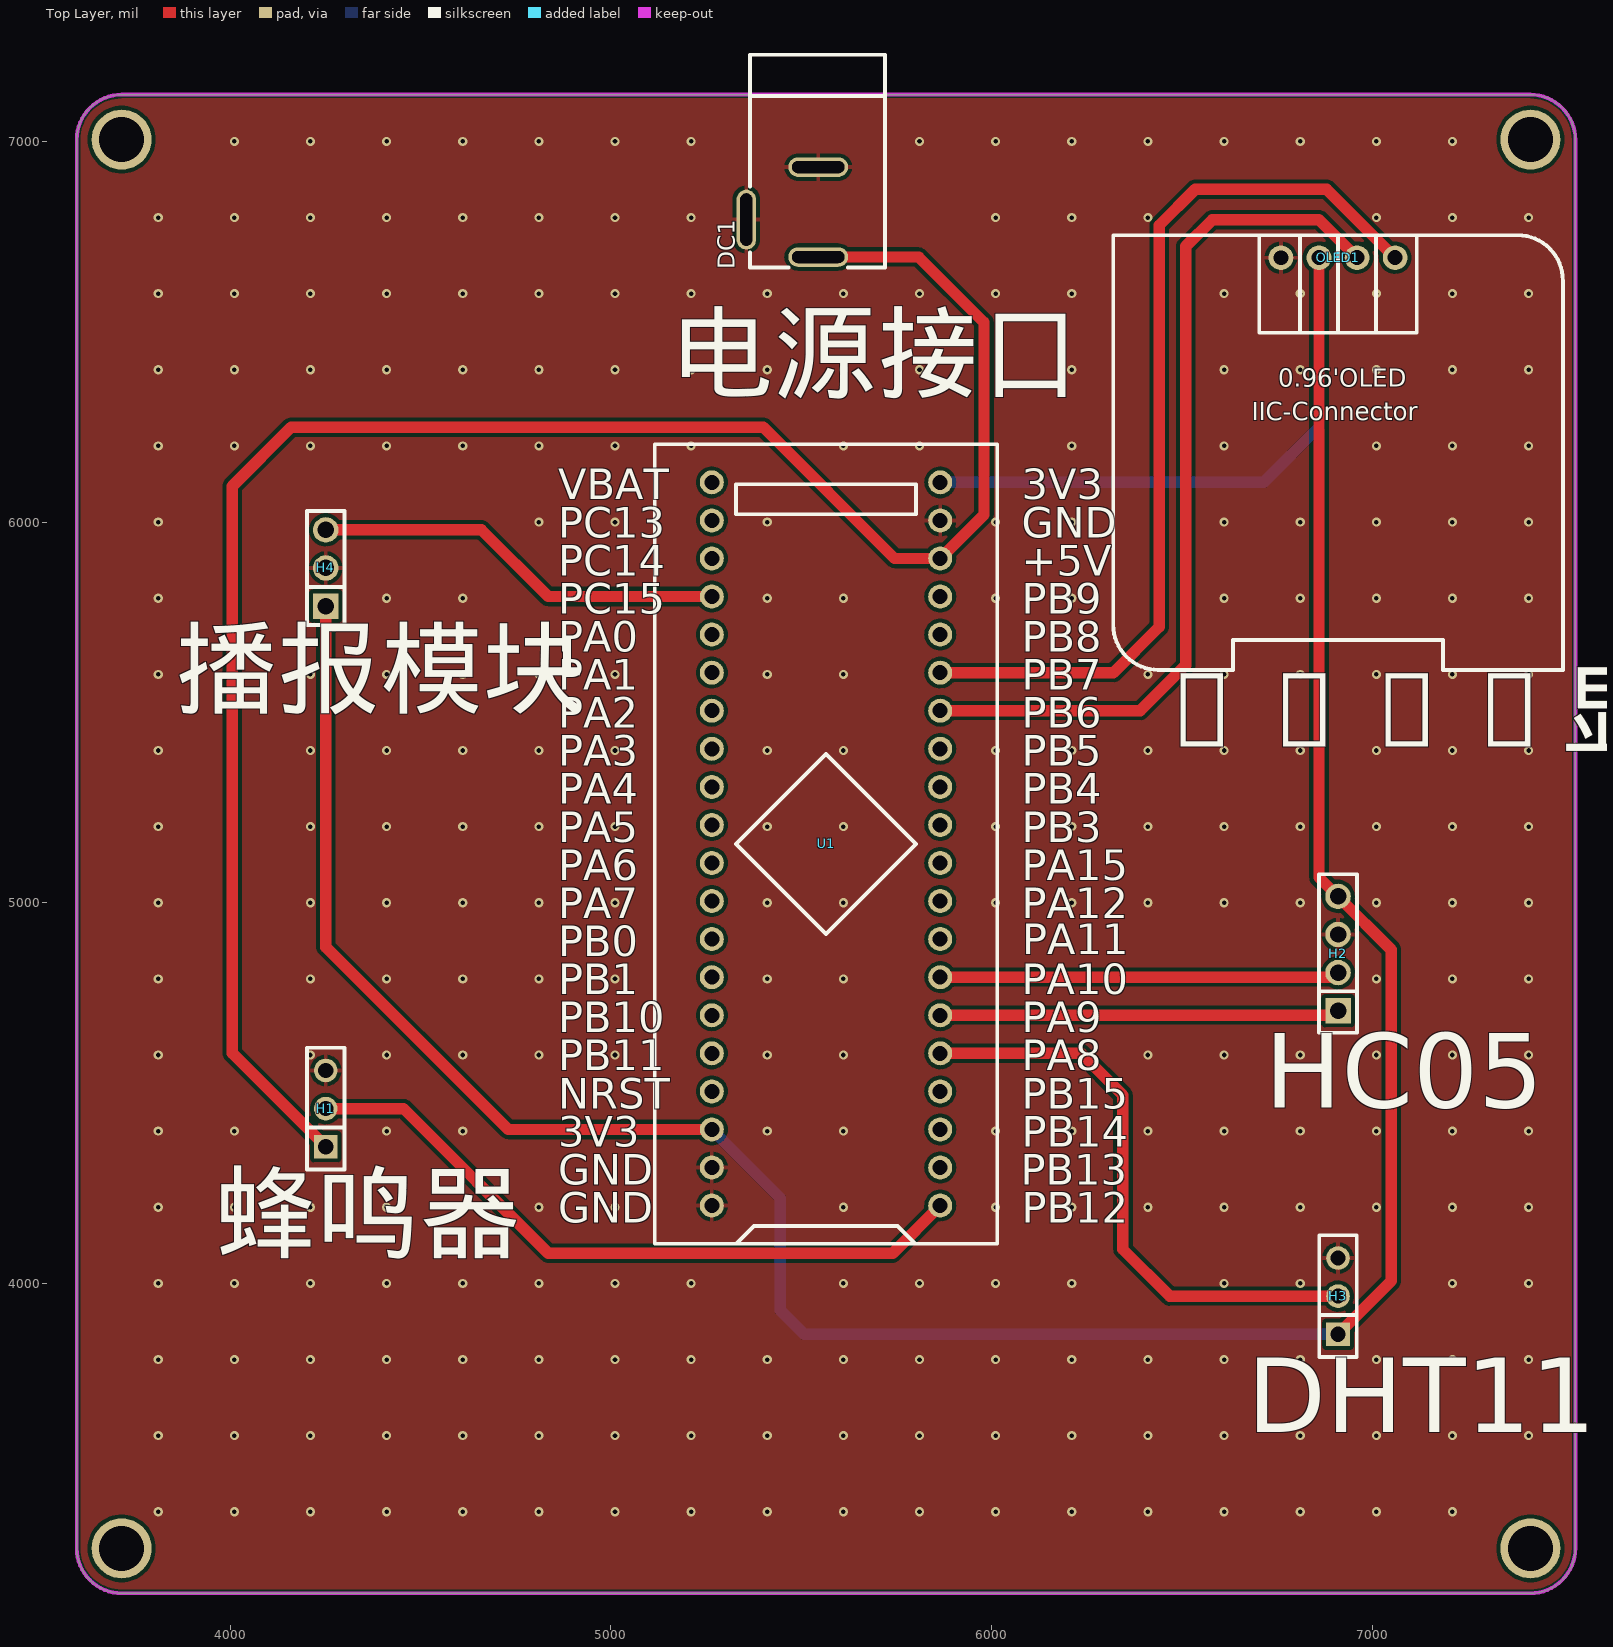
[diagram p0: Top Layer view]
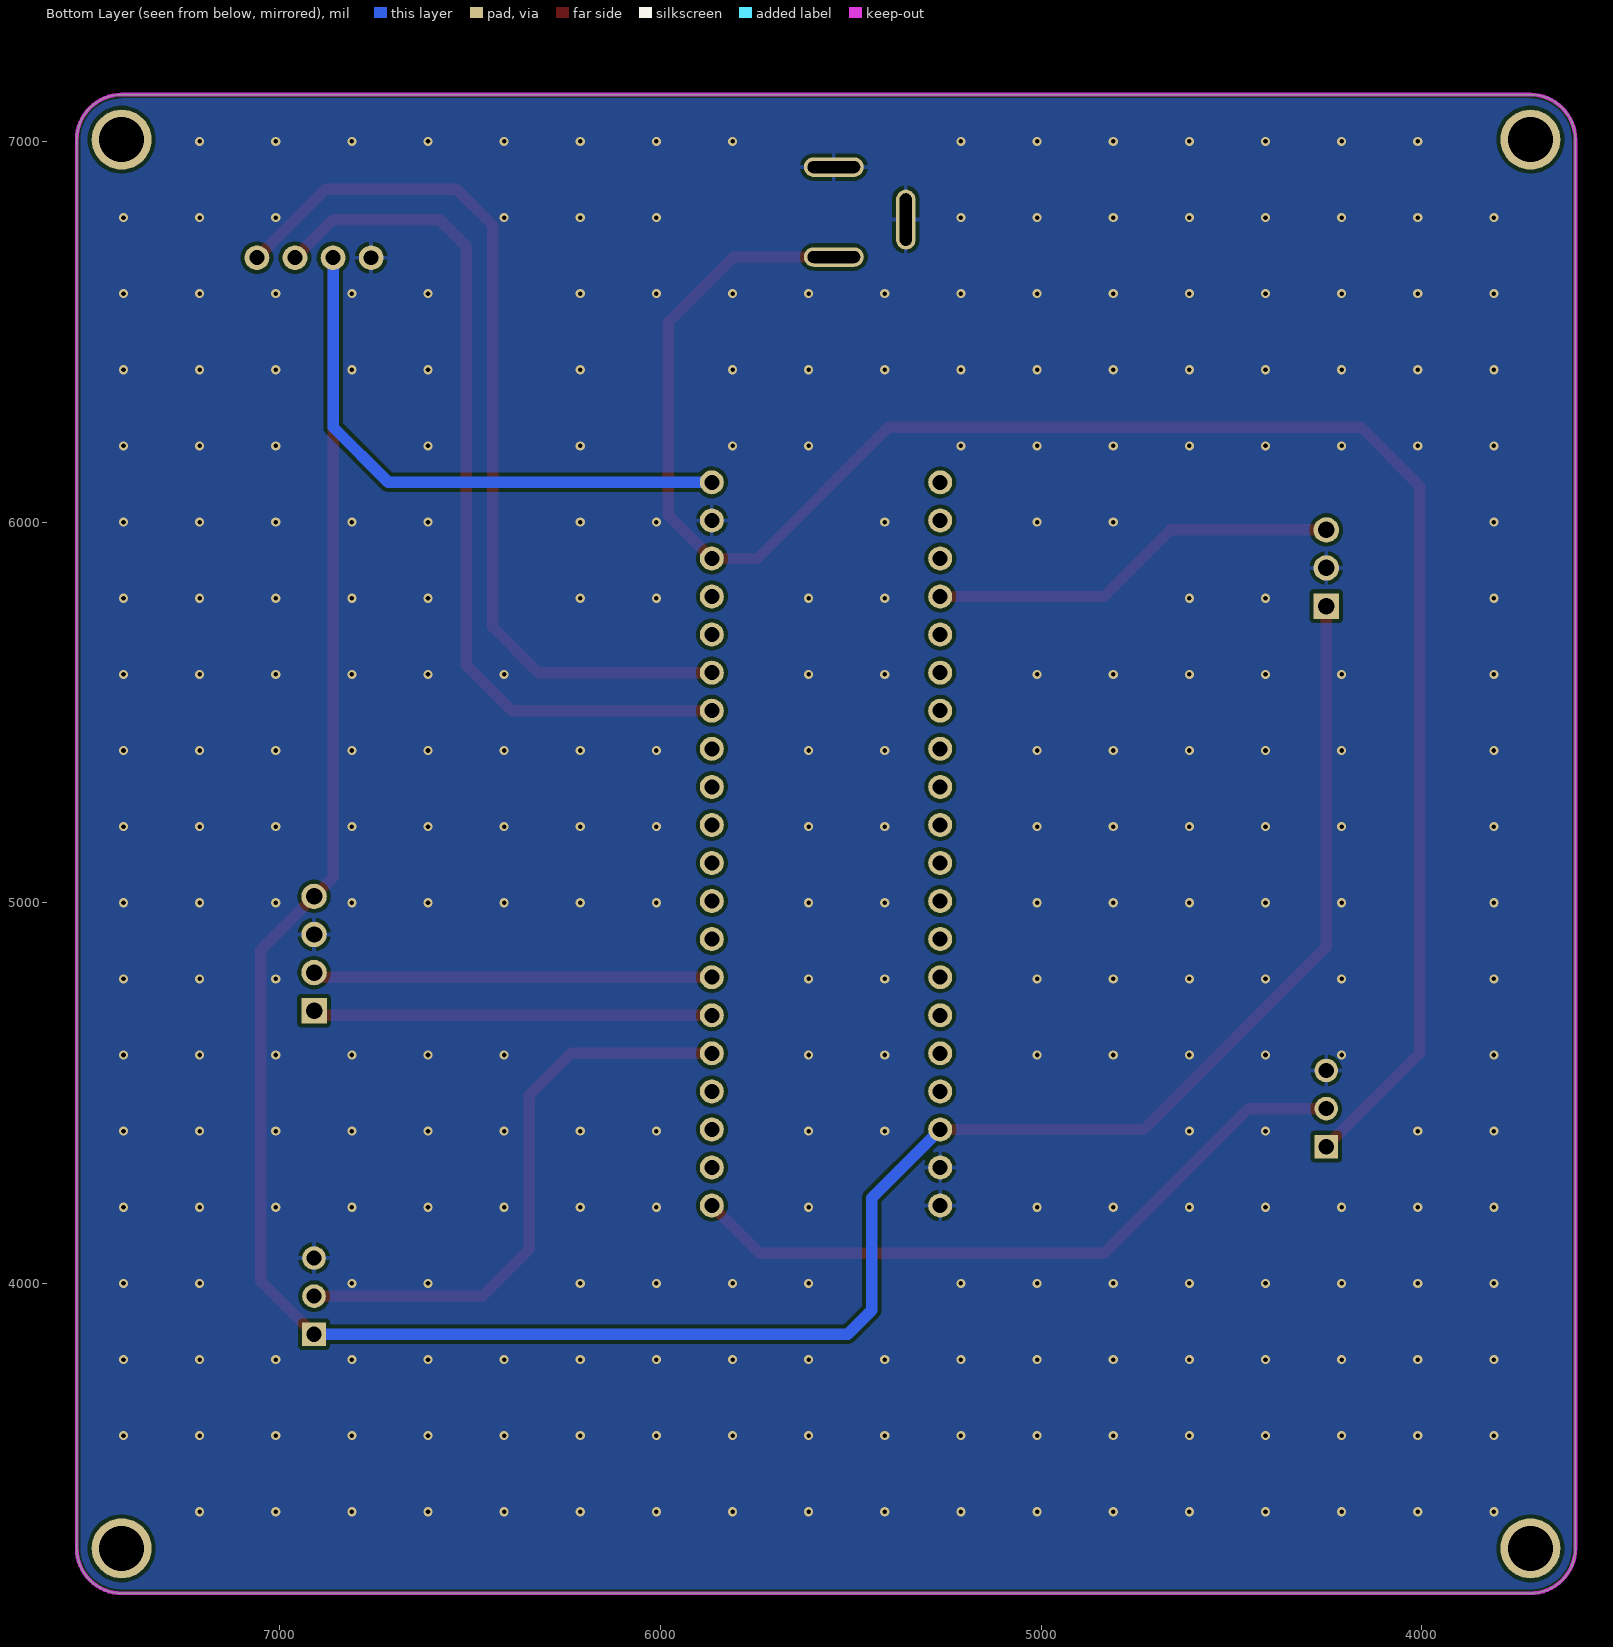
[diagram p1: Bottom Layer view, seen from below]
# Altium PCB MISC51802.pcbdoc
Units mil, origin at the board's own origin, x right, y up, seen from the top; angles counter-clockwise.
Board outline 3937.01 x 3937.01 mil, 2 copper layers (Top Layer, Bottom Layer), stack 62.206 mil thick; 7 components, 37 nets, 64 pads, 291 vias.

## Layer stack, top to bottom
Top Solder Mask Layer: solder mask 0.394, Dk 3.3
Top Layer: signal copper 1.379
Dielectric1: surface 59.449, FR4, Dk 4.5
Bottom Layer: signal copper 1.378
Bottom Solder Mask Layer: solder mask 0.394, Dk 3.3

## Board outline
3714.61,7123.5 ccw(c3714.61,7005.39) 3596.5,7005.39 3596.5,3304.61 ccw(c3714.61,3304.61) 3714.61,3186.5 7415.39,3186.5 ccw(c7415.39,3304.61) 7533.5,3304.61 7533.5,7005.39 ccw(c7415.39,7005.39) 7415.39,7123.5 3714.61,7123.5

## Design rules (kind name [scope] priority, off if disabled: settings)
BoardOutlineClearance copperThickness2oz_1 [All] p2 off: genericclearance=7.99 ignorepadtopadclearanceinfootprint=FALSE except(0: Arc-SplitContinuation Track-SplitContinuation SMDPad-SplitContinuation THPad-SplitContinuation Via-SplitContinuation Fill-SplitContinuation Region-SplitContinuation Poly-SplitContinuation Text-SplitContinuation Hole-SplitContinuation; 5.98: Arc-CutoutEdge Track-CutoutEdge SMDPad-CutoutEdge THPad-CutoutEdge Via-CutoutEdge Text-CutoutEdge; 6.9: Hole-OutlineEdge Hole-CutoutEdge; 10: Poly-OutlineEdge Poly-CutoutEdge; 11.81: Arc-OutlineEdge Track-OutlineEdge SMDPad-OutlineEdge THPad-OutlineEdge Via-OutlineEdge Fill-OutlineEdge Region-OutlineEdge Text-OutlineEdge Fill-CutoutEdge Region-CutoutEdge)
BoardOutlineClearance Plane_innerPlane_1 [All] p4 off: genericclearance=4.02 ignorepadtopadclearanceinfootprint=FALSE except(0: Arc-SplitContinuation Track-SplitContinuation SMDPad-SplitContinuation THPad-SplitContinuation Via-SplitContinuation Fill-SplitContinuation Region-SplitContinuation Poly-SplitContinuation Text-SplitContinuation Hole-SplitContinuation; 5.98: Arc-CutoutEdge Track-CutoutEdge SMDPad-CutoutEdge THPad-CutoutEdge Via-CutoutEdge Text-CutoutEdge; 6.9: Hole-OutlineEdge Hole-CutoutEdge; 10: Poly-OutlineEdge Poly-CutoutEdge; 11.81: Arc-OutlineEdge Track-OutlineEdge SMDPad-OutlineEdge THPad-OutlineEdge Via-OutlineEdge Fill-OutlineEdge Region-OutlineEdge Text-OutlineEdge Fill-CutoutEdge Region-CutoutEdge)
BoardOutlineClearance Copper_copperRegion_1 [All] p6 off: genericclearance=4.02 ignorepadtopadclearanceinfootprint=FALSE except(0: Arc-SplitContinuation Track-SplitContinuation SMDPad-SplitContinuation THPad-SplitContinuation Via-SplitContinuation Fill-SplitContinuation Region-SplitContinuation Poly-SplitContinuation Text-SplitContinuation Hole-SplitContinuation; 5.98: Arc-CutoutEdge Track-CutoutEdge SMDPad-CutoutEdge THPad-CutoutEdge Via-CutoutEdge Text-CutoutEdge; 6.9: Hole-OutlineEdge Hole-CutoutEdge; 10: Poly-OutlineEdge Poly-CutoutEdge; 11.81: Arc-OutlineEdge Track-OutlineEdge SMDPad-OutlineEdge THPad-OutlineEdge Via-OutlineEdge Fill-OutlineEdge Region-OutlineEdge Text-OutlineEdge Fill-CutoutEdge Region-CutoutEdge)
BoardOutlineClearance Copper_copperRegion_copperThickness1oz_1 [All] p8 off: genericclearance=4.02 ignorepadtopadclearanceinfootprint=FALSE except(0: Arc-SplitContinuation Track-SplitContinuation SMDPad-SplitContinuation THPad-SplitContinuation Via-SplitContinuation Fill-SplitContinuation Region-SplitContinuation Poly-SplitContinuation Text-SplitContinuation Hole-SplitContinuation; 5.98: Arc-CutoutEdge Track-CutoutEdge SMDPad-CutoutEdge THPad-CutoutEdge Via-CutoutEdge Text-CutoutEdge; 6.9: Hole-OutlineEdge Hole-CutoutEdge; 10: Poly-OutlineEdge Poly-CutoutEdge; 11.81: Arc-OutlineEdge Track-OutlineEdge SMDPad-OutlineEdge THPad-OutlineEdge Via-OutlineEdge Fill-OutlineEdge Region-OutlineEdge Text-OutlineEdge Fill-CutoutEdge Region-CutoutEdge)
BoardOutlineClearance Copper_copperRegion_Copper_copperRegion_1 [All] p10 off: genericclearance=4.02 ignorepadtopadclearanceinfootprint=FALSE except(0: Arc-SplitContinuation Track-SplitContinuation SMDPad-SplitContinuation THPad-SplitContinuation Via-SplitContinuation Fill-SplitContinuation Region-SplitContinuation Poly-SplitContinuation Text-SplitContinuation Hole-SplitContinuation; 5.98: Arc-CutoutEdge Track-CutoutEdge SMDPad-CutoutEdge THPad-CutoutEdge Via-CutoutEdge Text-CutoutEdge; 6.9: Hole-OutlineEdge Hole-CutoutEdge; 10: Poly-OutlineEdge Poly-CutoutEdge; 11.81: Arc-OutlineEdge Track-OutlineEdge SMDPad-OutlineEdge THPad-OutlineEdge Via-OutlineEdge Fill-OutlineEdge Region-OutlineEdge Text-OutlineEdge Fill-CutoutEdge Region-CutoutEdge)
BoardOutlineClearance copperThickness1oz_1 [All] p12: genericclearance=4.02 ignorepadtopadclearanceinfootprint=FALSE except(0: Arc-SplitContinuation Track-SplitContinuation SMDPad-SplitContinuation THPad-SplitContinuation Via-SplitContinuation Fill-SplitContinuation Region-SplitContinuation Poly-SplitContinuation Text-SplitContinuation Hole-SplitContinuation; 5.98: Arc-CutoutEdge Track-CutoutEdge SMDPad-CutoutEdge THPad-CutoutEdge Via-CutoutEdge Text-CutoutEdge; 6.9: Hole-OutlineEdge Hole-CutoutEdge; 10: Poly-OutlineEdge Poly-CutoutEdge; 11.81: Arc-OutlineEdge Track-OutlineEdge SMDPad-OutlineEdge THPad-OutlineEdge Via-OutlineEdge Fill-OutlineEdge Region-OutlineEdge Text-OutlineEdge Fill-CutoutEdge Region-CutoutEdge)
Clearance copperThickness2oz [All] p1 off: gap=7.99 ignorepadtopadclearanceinfootprint=FALSE except(5.98: SMDPad-Track SMDPad-SMDPad THPad-Track SMDPad-THPad THPad-THPad Track-Via SMDPad-Via THPad-Via Via-Via Fill-SMDPad Region-SMDPad Fill-THPad Region-THPad Fill-Via Region-Via Fill-Fill Fill-Region Region-Region Arc-Track Arc-SMDPad Arc-THPad Arc-Via Fill-Arc Region-Arc Arc-Arc Text-Track SMDPad-Text Text-THPad Text-Via Fill-Text Region-Text Arc-Text Text-Text; 6.9: Hole-Track Hole-SMDPad Hole-THPad Hole-Via Fill-Hole Region-Hole Hole-Arc Hole-Text; 10: Poly-Track Poly-SMDPad Poly-THPad Poly-Via Poly-Fill Poly-Region Poly-Poly Poly-Arc Poly-Text Poly-Hole; 11.81: Fill-Track Region-Track)
Clearance Plane_innerPlane [All] p3 off: gap=4.02 ignorepadtopadclearanceinfootprint=FALSE except(5.98: SMDPad-Track SMDPad-SMDPad THPad-Track SMDPad-THPad THPad-THPad Track-Via SMDPad-Via THPad-Via Via-Via Fill-SMDPad Region-SMDPad Fill-THPad Region-THPad Fill-Via Region-Via Fill-Fill Fill-Region Region-Region Arc-Track Arc-SMDPad Arc-THPad Arc-Via Fill-Arc Region-Arc Arc-Arc Text-Track SMDPad-Text Text-THPad Text-Via Fill-Text Region-Text Arc-Text Text-Text; 6.9: Hole-Track Hole-SMDPad Hole-THPad Hole-Via Fill-Hole Region-Hole Hole-Arc Hole-Text; 10: Poly-Track Poly-SMDPad Poly-THPad Poly-Via Poly-Fill Poly-Region Poly-Poly Poly-Arc Poly-Text Poly-Hole; 11.81: Fill-Track Region-Track)
Clearance Copper_copperRegion [All] p5 off: gap=4.02 ignorepadtopadclearanceinfootprint=FALSE except(5.98: SMDPad-Track SMDPad-SMDPad THPad-Track SMDPad-THPad THPad-THPad Track-Via SMDPad-Via THPad-Via Via-Via Fill-SMDPad Region-SMDPad Fill-THPad Region-THPad Fill-Via Region-Via Fill-Fill Fill-Region Region-Region Arc-Track Arc-SMDPad Arc-THPad Arc-Via Fill-Arc Region-Arc Arc-Arc Text-Track SMDPad-Text Text-THPad Text-Via Fill-Text Region-Text Arc-Text Text-Text; 6.9: Hole-Track Hole-SMDPad Hole-THPad Hole-Via Fill-Hole Region-Hole Hole-Arc Hole-Text; 10: Poly-Track Poly-SMDPad Poly-THPad Poly-Via Poly-Fill Poly-Region Poly-Poly Poly-Arc Poly-Text Poly-Hole; 11.81: Fill-Track Region-Track)
Clearance Copper_copperRegion_copperThickness1oz [All] p7 off: gap=4.02 ignorepadtopadclearanceinfootprint=FALSE except(5.98: SMDPad-Track SMDPad-SMDPad THPad-Track SMDPad-THPad THPad-THPad Track-Via SMDPad-Via THPad-Via Via-Via Fill-SMDPad Region-SMDPad Fill-THPad Region-THPad Fill-Via Region-Via Fill-Fill Fill-Region Region-Region Arc-Track Arc-SMDPad Arc-THPad Arc-Via Fill-Arc Region-Arc Arc-Arc Text-Track SMDPad-Text Text-THPad Text-Via Fill-Text Region-Text Arc-Text Text-Text; 6.9: Hole-Track Hole-SMDPad Hole-THPad Hole-Via Fill-Hole Region-Hole Hole-Arc Hole-Text; 10: Poly-Track Poly-SMDPad Poly-THPad Poly-Via Poly-Fill Poly-Region Poly-Poly Poly-Arc Poly-Text Poly-Hole; 11.81: Fill-Track Region-Track)
Clearance Copper_copperRegion_Copper_copperRegion [All] p9 off: gap=4.02 ignorepadtopadclearanceinfootprint=FALSE except(5.98: SMDPad-Track SMDPad-SMDPad THPad-Track SMDPad-THPad THPad-THPad Track-Via SMDPad-Via THPad-Via Via-Via Fill-SMDPad Region-SMDPad Fill-THPad Region-THPad Fill-Via Region-Via Fill-Fill Fill-Region Region-Region Arc-Track Arc-SMDPad Arc-THPad Arc-Via Fill-Arc Region-Arc Arc-Arc Text-Track SMDPad-Text Text-THPad Text-Via Fill-Text Region-Text Arc-Text Text-Text; 6.9: Hole-Track Hole-SMDPad Hole-THPad Hole-Via Fill-Hole Region-Hole Hole-Arc Hole-Text; 10: Poly-Track Poly-SMDPad Poly-THPad Poly-Via Poly-Fill Poly-Region Poly-Poly Poly-Arc Poly-Text Poly-Hole; 11.81: Fill-Track Region-Track)
Clearance copperThickness1oz [All] p11: gap=4.02 ignorepadtopadclearanceinfootprint=FALSE except(5.98: SMDPad-Track SMDPad-SMDPad THPad-Track SMDPad-THPad THPad-THPad Track-Via SMDPad-Via THPad-Via Via-Via Fill-SMDPad Region-SMDPad Fill-THPad Region-THPad Fill-Via Region-Via Fill-Fill Fill-Region Region-Region Arc-Track Arc-SMDPad Arc-THPad Arc-Via Fill-Arc Region-Arc Arc-Arc Text-Track SMDPad-Text Text-THPad Text-Via Fill-Text Region-Text Arc-Text Text-Text; 6.9: Hole-Track Hole-SMDPad Hole-THPad Hole-Via Fill-Hole Region-Hole Hole-Arc Hole-Text; 10: Poly-Track Poly-SMDPad Poly-THPad Poly-Via Poly-Fill Poly-Region Poly-Poly Poly-Arc Poly-Text Poly-Hole; 11.81: Fill-Track Region-Track)
DiffPairsRouting differentialPair [All] p1: maxlimit=6 minlimit=6 mostfreqgap=6 toplayer_minwidth=5 toplayer_prefwidth=10 toplayer_maxwidth=100 toplayer_mingap=6 toplayer_prefgap=6 toplayer_maxgap=6 bottomlayer_minwidth=5 bottomlayer_prefwidth=10 bottomlayer_maxwidth=100 bottomlayer_mingap=6 bottomlayer_prefgap=6 bottomlayer_maxgap=6 maxuncoupledlength=10
HoleToHoleClearance otherClearance [All] p1: gap=11.81 allowstackedmicrovias=TRUE
Length netLength [All] p1: minlimit=0 maxlimit=0
PasteMaskExpansion pasteMaskExpansion [All] p1: expansion=0
PlaneConnect innerPlane [All] p1: planeconnectstyle=Relief reliefexpansion=20 reliefentries=4 reliefconductorwidth=10 reliefairgap=10
PolygonConnect copperRegion_copperThickness1oz [All] p1 off: connectstyle=Relief reliefconductorwidth=10 reliefentries=4 polygonreliefangle="90 Angle" airgapwidth=10 via.connectstyle=Relief via.reliefconductorwidth=10 via.reliefentries=4 via.polygonreliefangle="90 Angle" via.airgapwidth=10
PolygonConnect copperRegion_Copper_copperRegion [All] p2 off: connectstyle=Relief reliefconductorwidth=10 reliefentries=4 polygonreliefangle="90 Angle" airgapwidth=10 via.connectstyle=Relief via.reliefconductorwidth=10 via.reliefentries=4 via.polygonreliefangle="90 Angle" via.airgapwidth=10
PolygonConnect copperRegion [All] p3: connectstyle=Relief reliefconductorwidth=10 reliefentries=4 polygonreliefangle="90 Angle" airgapwidth=10 via.connectstyle=Relief via.reliefconductorwidth=10 via.reliefentries=4 via.polygonreliefangle="90 Angle" via.airgapwidth=10
RoutingVias viaSize [All] p1: holewidth=12.01 width=24.02 viastyle="Through Hole" minholewidth=11.81 minwidth=19.68 maxholewidth=248.03 maxwidth=393.7
SolderMaskExpansion solderMaskExpansion [IsVia] p1: expansion=-1000 istentingtop=TRUE
SolderMaskExpansion solderMaskExpansion [All] p2: expansion=2 istentingtop=FALSE
Width copperThickness2oz_2 [All] p1 off: maxlimit=100 minlimit=8 preferedwidth=10
Width copperThickness1oz_2 [All] p2: maxlimit=100 minlimit=5 preferedwidth=10

## Components (designator, comment, footprint, x,y, rotation, side; value= is the part's Value field where it differs from the comment)
DC1 "" DC-2.0 5555,6820 r90 top
H1 "" HDR-TH_3P-P2.54-V-F 4250.79,4459.92 r90 top
H2 "" HDR-TH_4P-P2.54-V-F 6910,4867.19 r90 top
H3 "" HDR-TH_3P-P2.54-V-F 6910,3967.24 r90 top
H4 "" HDR-TH_3P-P2.54-V-M 4250.79,5880 r90 top
OLED1 "" 0.96OLED_4P 6910,6695 r0 top
U1 "STM32F103C8T6-Card" CONN-TH_L53.3-W22.9_STM32F103C8T6-CARD 5565,5155 r90 top

## Footprints (in the part's own frame and the unit in brackets; to place one, negate y for a bottom-side part, rotate by r counter-clockwise, add the part's x,y. Pads: shape width x height; smd on the part's side, far side on the other; paste and mask are expansions set on the pad)
0.96OLED_4P [mm]
  round 1.65 hole 1 copper offset 0,0: 1(-3.81,-0.001) 2(-1.27,0.002) 3(1.27,0.002) 4(3.81,0.002)
  silkscreen extent -15,-27.5 15,1.5
CONN-TH_L53.3-W22.9_STM32F103C8T6-CARD [mm]
  round 1.6 hole 1: 1(-24.13,-7.62) 2(-21.59,-7.62) 3(-19.05,-7.62) 4(-16.51,-7.62) 5(-13.97,-7.62) 6(-11.43,-7.62) 7(-8.89,-7.62) 8(-6.35,-7.62) 9(-3.81,-7.62) 10(-1.27,-7.62) 11(1.27,-7.62) 12(3.81,-7.62) 13(6.35,-7.62) 14(8.89,-7.62) 15(11.43,-7.62) 16(13.97,-7.62) 17(16.51,-7.62) 18(19.05,-7.62) 19(21.59,-7.62) 20(24.13,-7.62) 21(24.13,7.62) 22(21.59,7.62) 23(19.05,7.62) 24(16.51,7.62) 25(13.97,7.62) 26(11.43,7.62) 27(8.89,7.62) 28(6.35,7.62) 29(3.81,7.62) 30(1.27,7.62) 31(-1.27,7.62) 32(-3.81,7.62) 33(-6.35,7.62) 34(-8.89,7.62) 35(-11.43,7.62) 36(-13.97,7.62) 37(-16.51,7.62) 38(-19.05,7.62) 39(-21.59,7.62) 40(-24.13,7.62)
  silkscreen extent -26.67,-11.43 26.67,11.43
DC-2.0 [mil]
  oval 157.5x51.2 hole 31.5 slot 137.8 at 0 deg paste+0 mask+2: 2(-24.7,199.5)
  oval 51.2x157.5 hole 31.5 slot 137.8 at 90 deg paste+0 mask+2: 3(113.1,10.5) 4(-123.1,10.5)
  silkscreen extent -151,-165 408,190
HDR-TH_3P-P2.54-V-F [mil]
  rect 62x62 hole 40.16: 1(-100,0)
  round 62 hole 40.16: 2(0,0) 3(100,0)
  silkscreen extent -160,-49 160,49
HDR-TH_3P-P2.54-V-M [mm]
  rect 1.7x1.7 hole 1.1: 1(-2.54,0)
  round 1.7 hole 1.1: 2(0,0) 3(2.54,0)
  silkscreen extent -3.81,-1.25 3.81,1.25
HDR-TH_4P-P2.54-V-F [mm]
  rect 1.7x1.7 hole 1.1: 1(-3.81,0)
  round 1.7 hole 1.1: 2(-1.27,0) 3(1.27,0) 4(3.81,0)
  silkscreen extent -5.29,-1.27 5.29,1.27

## Free pads (board coordinates)
  round 157.48 hole 118.11: 1(3714.61,7005.39) 1(3714.61,3304.61) 1(7415.39,7005.39) 1(7415.39,3304.61)

## Via types
v1: diameter 24.02, hole 12, Top Layer to Bottom Layer, 291 vias

## Nets (pads, with @x,y where several pads share a name; then routed paths per layer and width w, separated by ;. In a path a pad name is that pad's centre, name@x,y a point inside that pad or via, vN(x,y) a via of type N, cw(c..) or ccw(c..) an arc to the next point about the centre after c; other vN are vias at no path point)
+5V: DC1.4 H1.1 U1.18 | length 5078.3
  Top Layer w30: H1.1 4005,4605.71 4005,6095 4160,6250 5400,6250 5745,5905 U1.18 5980,6020 5980,6525 5808.1,6696.9 DC1.4
GND: DC1.2 DC1.3 H1.3 H2.3 H3.3 H4.2 OLED1.1 U1.19 U1.39 U1.40
  other v1: 3810.6,3400.6 4010.6,3400.6 4210.6,3400.6 4410.6,3400.6 4610.6,3400.6 4810.6,3400.6 5010.6,3400.6 5210.6,3400.6 5410.6,3400.6 5610.6,3400.6 5810.6,3400.6 6010.6,3400.6 6210.6,3400.6 6410.6,3400.6 6610.6,3400.6 6810.6,3400.6 7010.6,3400.6 7210.6,3400.6 3810.6,3600.6 4010.6,3600.6 4210.6,3600.6 4410.6,3600.6 4610.6,3600.6 4810.6,3600.6 5010.6,3600.6 5210.6,3600.6 5410.6,3600.6 5610.6,3600.6 5810.6,3600.6 6010.6,3600.6 6210.6,3600.6 6410.6,3600.6 6610.6,3600.6 6810.6,3600.6 7010.6,3600.6 7210.6,3600.6 7410.6,3600.6 3810.6,3800.6 4010.6,3800.6 4210.6,3800.6 4410.6,3800.6 4610.6,3800.6 4810.6,3800.6 5010.6,3800.6 5210.6,3800.6 5410.6,3800.6 5610.6,3800.6 5810.6,3800.6 6010.6,3800.6 6210.6,3800.6 6410.6,3800.6 6610.6,3800.6 6810.6,3800.6 7010.6,3800.6 7210.6,3800.6 7410.6,3800.6 3810.6,4000.6 4010.6,4000.6 4210.6,4000.6 4410.6,4000.6 4610.6,4000.6 4810.6,4000.6 5010.6,4000.6 5210.6,4000.6 5610.6,4000.6 5810.6,4000.6 6010.6,4000.6 6210.6,4000.6 6610.6,4000.6 6810.6,4000.6 7210.6,4000.6 7410.6,4000.6 3810.6,4200.6 4010.6,4200.6 4210.6,4200.6 4410.6,4200.6 4610.6,4200.6 4810.6,4200.6 5010.6,4200.6 5610.6,4200.6 6010.6,4200.6 6210.6,4200.6 6410.6,4200.6 6610.6,4200.6 6810.6,4200.6 7010.6,4200.6 7210.6,4200.6 7410.6,4200.6 3810.6,4400.6 4010.6,4400.6 4410.6,4400.6 4610.6,4400.6 5410.6,4400.6 5610.6,4400.6 6010.6,4400.6 6210.6,4400.6 6410.6,4400.6 6610.6,4400.6 6810.6,4400.6 7010.6,4400.6 7210.6,4400.6 7410.6,4400.6 3810.6,4600.6 4210.6,4600.6 4410.6,4600.6 4610.6,4600.6 4810.6,4600.6 5010.6,4600.6 5410.6,4600.6 5610.6,4600.6 6410.6,4600.6 6610.6,4600.6 6810.6,4600.6 7010.6,4600.6 7210.6,4600.6 7410.6,4600.6 3810.6,4800.6 4210.6,4800.6 4410.6,4800.6 4610.6,4800.6 4810.6,4800.6 5010.6,4800.6 5410.6,4800.6 5610.6,4800.6 7010.6,4800.6 7210.6,4800.6 7410.6,4800.6 3810.6,5000.6 4210.6,5000.6 4410.6,5000.6 4610.6,5000.6 4810.6,5000.6 5010.6,5000.6 5410.6,5000.6 5610.6,5000.6 6010.6,5000.6 6210.6,5000.6 6410.6,5000.6 6610.6,5000.6 6810.6,5000.6 7010.6,5000.6 7210.6,5000.6 7410.6,5000.6 3810.6,5200.6 4210.6,5200.6 4410.6,5200.6 4610.6,5200.6 4810.6,5200.6 5010.6,5200.6 5410.6,5200.6 5610.6,5200.6 6010.6,5200.6 6210.6,5200.6 6410.6,5200.6 6610.6,5200.6 6810.6,5200.6 7010.6,5200.6 7210.6,5200.6 7410.6,5200.6 3810.6,5400.6 4210.6,5400.6 4410.6,5400.6 4610.6,5400.6 4810.6,5400.6 5010.6,5400.6 5410.6,5400.6 5610.6,5400.6 6010.6,5400.6 6210.6,5400.6 6410.6,5400.6 6610.6,5400.6 6810.6,5400.6 7010.6,5400.6 7210.6,5400.6 7410.6,5400.6 3810.6,5600.6 4210.6,5600.6 4410.6,5600.6 4610.6,5600.6 4810.6,5600.6 5010.6,5600.6 5410.6,5600.6 5610.6,5600.6 6410.6,5600.6 6610.6,5600.6 6810.6,5600.6 7010.6,5600.6 7210.6,5600.6 7410.6,5600.6 3810.6,5800.6 4410.6,5800.6 4610.6,5800.6 5410.6,5800.6 5610.6,5800.6 6010.6,5800.6 6210.6,5800.6 6610.6,5800.6 6810.6,5800.6 7010.6,5800.6 7210.6,5800.6 7410.6,5800.6 3810.6,6000.6 4810.6,6000.6 5010.6,6000.6 5410.6,6000.6 6010.6,6000.6 6210.6,6000.6 6610.6,6000.6 6810.6,6000.6 7010.6,6000.6 7210.6,6000.6 7410.6,6000.6 3810.6,6200.6 4010.6,6200.6 4210.6,6200.6 4410.6,6200.6 4610.6,6200.6 4810.6,6200.6 5010.6,6200.6 5210.6,6200.6 5610.6,6200.6 5810.6,6200.6 6210.6,6200.6 6610.6,6200.6 7010.6,6200.6 7210.6,6200.6 7410.6,6200.6 3810.6,6400.6 4010.6,6400.6 4210.6,6400.6 4410.6,6400.6 4610.6,6400.6 4810.6,6400.6 5010.6,6400.6 5210.6,6400.6 5410.6,6400.6 5610.6,6400.6 5810.6,6400.6 6210.6,6400.6 6610.6,6400.6 6810.6,6400.6 7010.6,6400.6 7210.6,6400.6 7410.6,6400.6 3810.6,6600.6 4010.6,6600.6 4210.6,6600.6 4410.6,6600.6 4610.6,6600.6 4810.6,6600.6 5010.6,6600.6 5210.6,6600.6 5410.6,6600.6 5610.6,6600.6 5810.6,6600.6 6010.6,6600.6 6210.6,6600.6 6610.6,6600.6 6810.6,6600.6 7010.6,6600.6 7210.6,6600.6 7410.6,6600.6 3810.6,6800.6 4010.6,6800.6 4210.6,6800.6 4410.6,6800.6 4610.6,6800.6 4810.6,6800.6 5010.6,6800.6 5210.6,6800.6 6010.6,6800.6 6210.6,6800.6 6410.6,6800.6 7010.6,6800.6 7210.6,6800.6 7410.6,6800.6 4010.6,7000.6 4210.6,7000.6 4410.6,7000.6 4610.6,7000.6 4810.6,7000.6 5010.6,7000.6 5210.6,7000.6 5810.6,7000.6 6010.6,7000.6 6210.6,7000.6 6410.6,7000.6 6610.6,7000.6 6810.6,7000.6 7010.6,7000.6 7210.6,7000.6
NRST: U1.37
PA0: U1.25
PA1: U1.26
PA2: U1.27
PA3: U1.28
PA4: U1.29
PA5: U1.30
PA6: U1.31
PA7: U1.32
PA8: H3.2 U1.5 | length 1546.4
  Top Layer w30: U1.5 6235,4605 6345,4495 6345,4090 6467.76,3967.24 H3.2
PA9: H2.1 U1.6 | length 1050
  Top Layer w30: U1.6 6897.81,4705 H2.1
PA10: H2.2 U1.7 | length 1050
  Top Layer w30: U1.7 6897.81,4805 H2.2
PA11: U1.8
PA12: U1.9
PA15: U1.10
PB0: U1.33
PB1: U1.34
PB3: U1.11
PB4: U1.12
PB5: U1.13
PB6: OLED1.3 U1.14 | length 2315.1
  Top Layer w30: U1.14 6390,5505 6510,5625 6510,6725 6580,6795 6860.05,6795 OLED1.3@6960,6695.05
PB7: OLED1.4 U1.15 | length 2413.6
  Top Layer w30: U1.15 6320,5605 6440,5725 6440,6780 6535,6875 6880.05,6875 OLED1.4@7060,6695.05
PB8: U1.16
PB9: U1.17
PB10: U1.35
PB11: U1.36
PB12: H1.2 U1.1 | length 1823.4
  Top Layer w30: H1.2 4455.08,4459.92 4835,4080 5740,4080 U1.1
PB13: U1.2
PB14: U1.3
PB15: U1.4
PC13: U1.22
PC14: U1.23
PC15: H4.3 U1.24 | length 1086.7
  Top Layer w30: H4.3 4660,5980 4835,5805 U1.24
VBAT: U1.21
VCC: H2.4 H3.1 H4.1 OLED1.2 U1.20 U1.38 | length 8613.7
  Top Layer w30: H4.1 4250.79,4884.21 4730,4405 U1.38 ; OLED1.2@6860,6695.05 6860,5067.18 H2.4 7050,4877.18 7050,4007.25 H3.1
  Bottom Layer w30: U1.38 5445,4225 5445,3930 5507.76,3867.24 H3.1 ; U1.20 6715,6105 6860,6250 OLED1.2@6860,6695.05

## Polygon pours and split planes (outlines as drawn)
GND on Bottom Layer (solid, remove dead copper, pour order 2): 3525,7245 3525,3080 7700,3080 7700,7245
GND on Top Layer (solid, remove dead copper, pour order 2): 3000,7415 3000,3000 7930,3000 7930,7415

## Keep-outs
Board Outline Layer:
  the board outline again, w10

## Silkscreen, mask and mechanical layers (free items; w line width, h text height)
Top Silkscreen Layer:
  text "电源接口" at 5160,6350 h196.85
  text "VBAT" at 4860.95,6060 h80
  text "3V3" at 6079.16,6060 h80
  text "PC13" at 4860.95,5960 h80
  text "GND" at 6079.16,5960 h80
  text "PC14" at 4860.95,5860 h80
  text "+5V" at 6079.16,5860 h80
  text "PC15" at 4860.95,5760 h80
  text "PB9" at 6079.16,5760 h80
  text "PA0" at 4860.95,5660 h80
  text "PB8" at 6079.16,5660 h80
  text "PA1" at 4860.95,5560 h80
  text "PB7" at 6079.16,5560 h80
  text "播报模块" at 3855.48,5520.52 h196.85
  text "PA2" at 4860.95,5460 h80
  text "PB6" at 6079.16,5460 h80
  text "Oled显示器" at 6418.02,5410.48 h196.85
  text "PA3" at 4860.95,5360 h80
  text "PB5" at 6079.16,5360 h80
  text "PA4" at 4860.95,5260 h80
  text "PB4" at 6079.16,5260 h80
  text "PA5" at 4860.95,5160 h80
  text "PB3" at 6079.16,5160 h80
  text "PA6" at 4860.95,5060 h80
  text "PA15" at 6079.16,5060 h80
  text "PA7" at 4860.95,4960 h80
  text "PA12" at 6079.16,4960 h80
  text "PA11" at 6080.95,4865 h80
  text "PB0" at 4860.95,4860 h80
  text "PB1" at 4860.95,4760 h80
  text "PA10" at 6079.16,4760 h80
  text "PB10" at 4860.95,4660 h80
  text "PA9" at 6079.16,4660 h80
  text "PB11" at 4860.95,4560 h80
  text "PA8" at 6079.16,4560 h80
  text "HC05" at 6717.92,4461.52 h196.85
  text "NRST" at 4860.95,4460 h80
  text "PB15" at 6079.16,4460 h80
  text "3V3" at 4860.95,4360 h80
  text "PB14" at 6079.16,4360 h80
  text "GND" at 4860.95,4260 h80
  text "PB13" at 6075.95,4260 h80
  text "GND" at 4860.95,4160 h80
  text "PB12" at 6079.16,4160 h80
  text "蜂鸣器" at 3957.6,4090 h196.85
  text "DHT11" at 6671.39,3610 h196.85